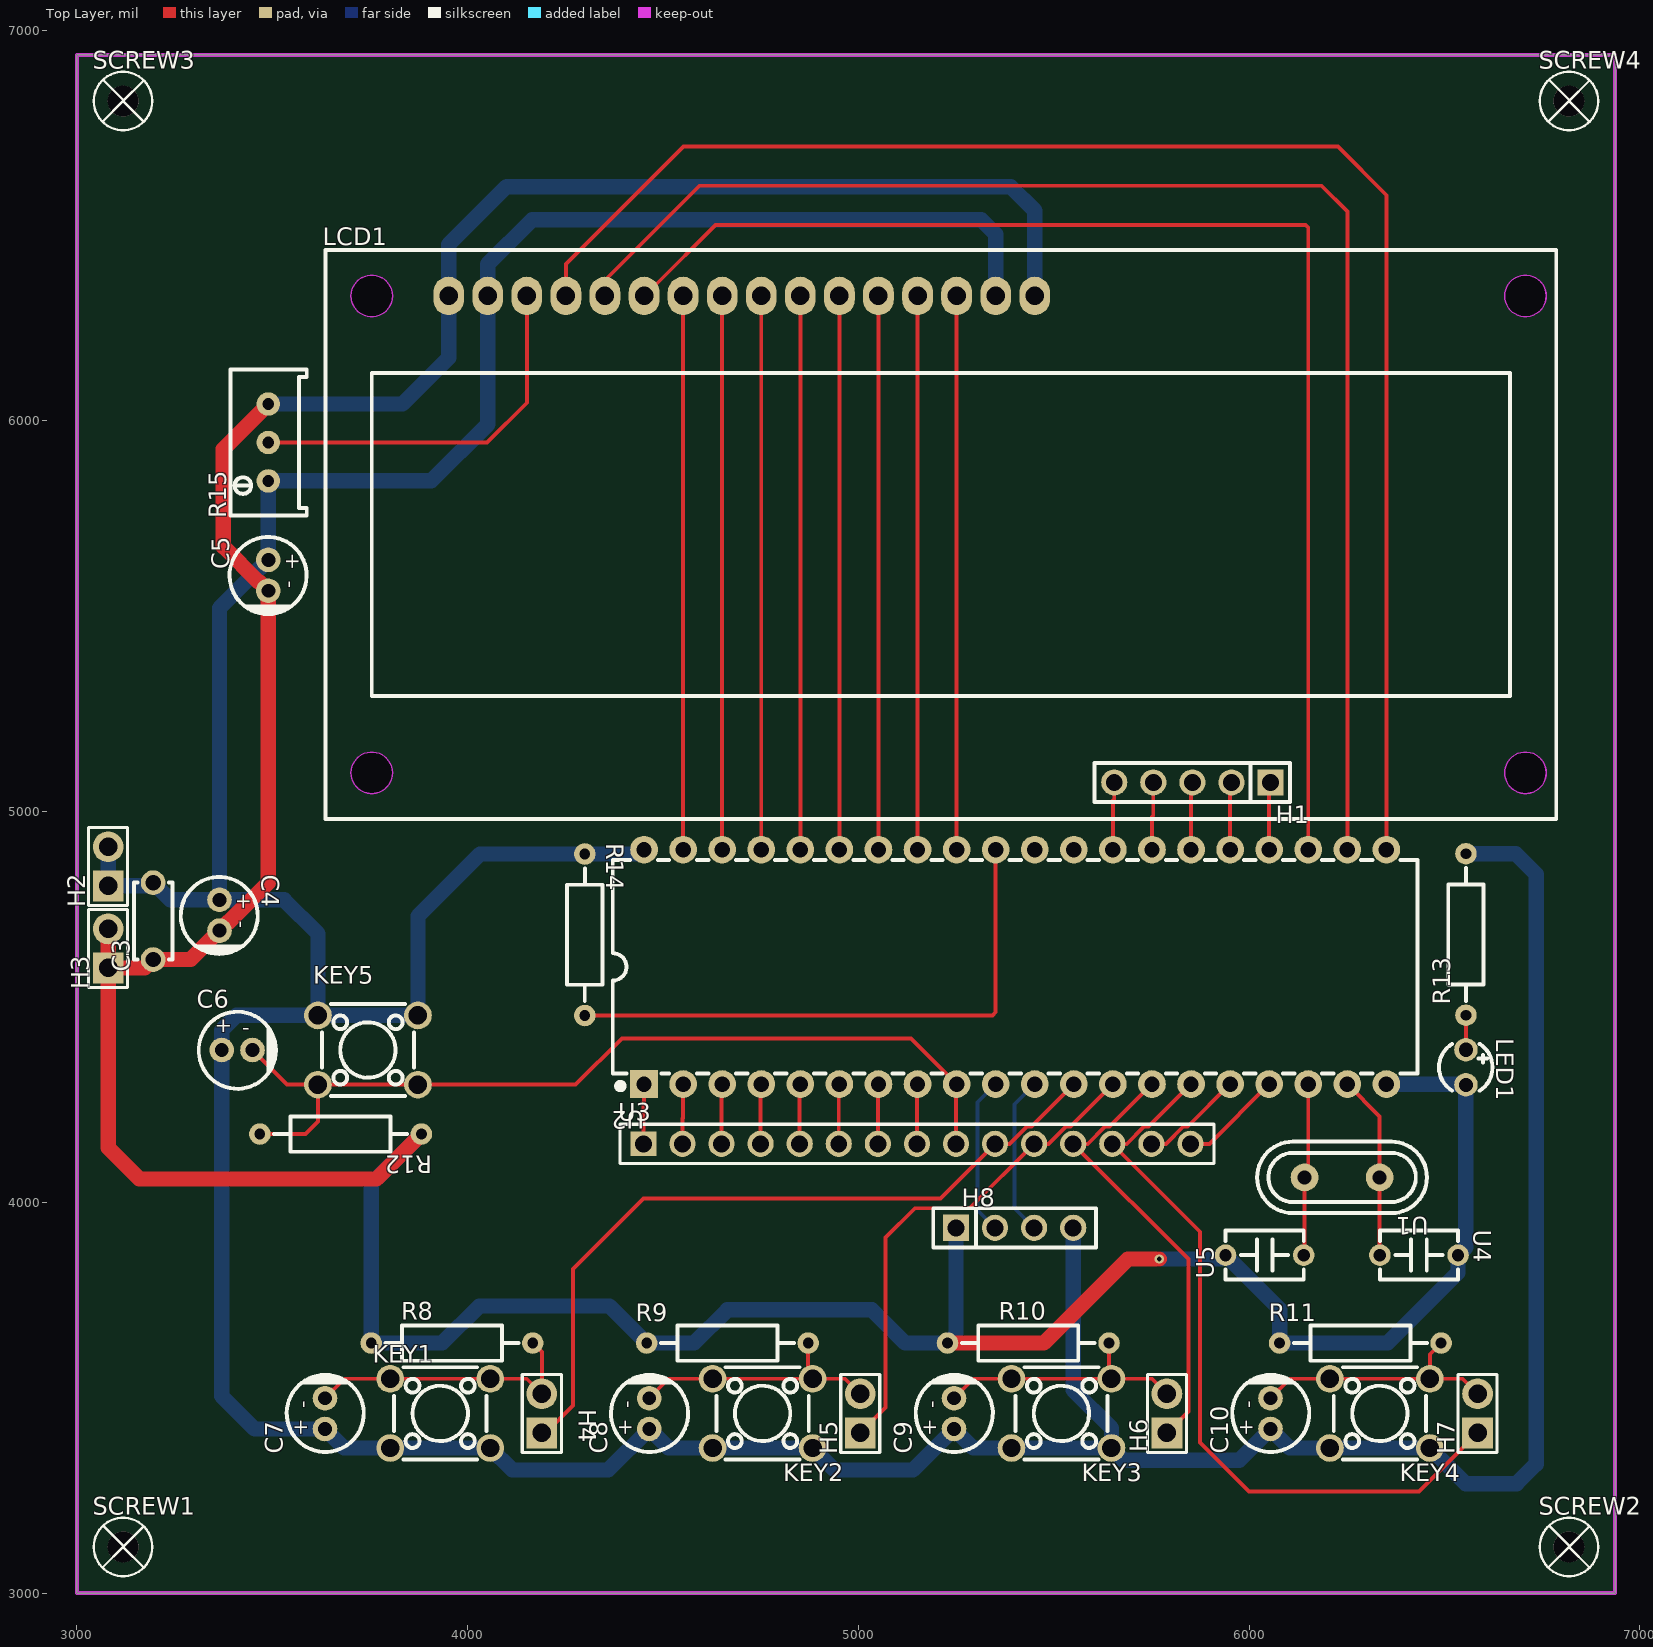
[diagram p0: Top Layer view]
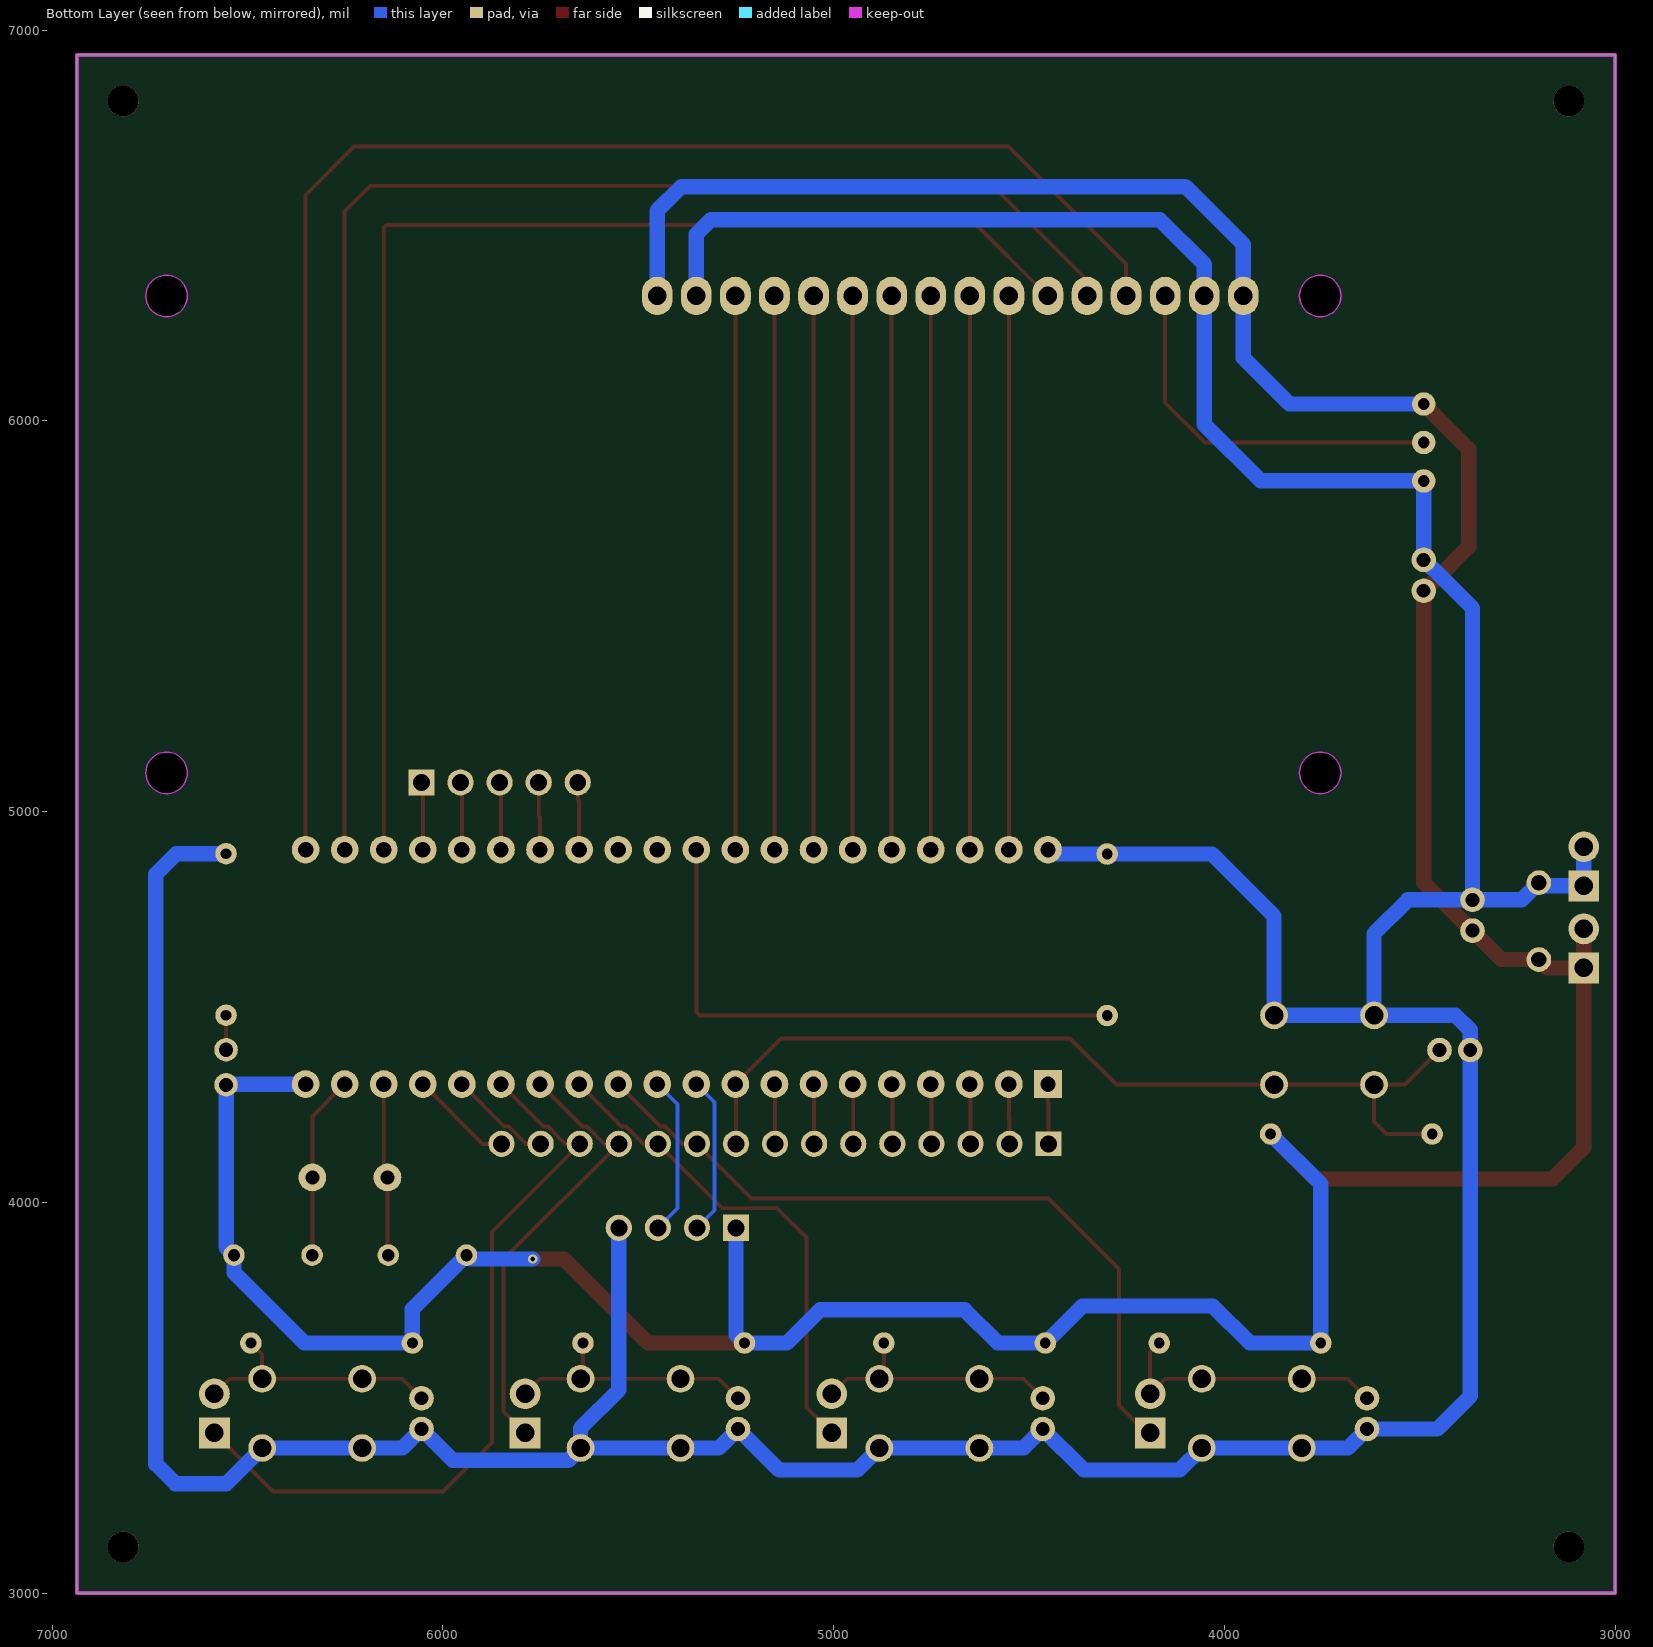
[diagram p1: Bottom Layer view, seen from below]
# Altium PCB MISC52019.pcbdoc
Units mil, origin at the board's own origin, x right, y up, seen from the top; angles counter-clockwise.
Board outline 3937.01 x 3937.01 mil, 2 copper layers (Top Layer, Bottom Layer), stack 62.206 mil thick; 40 components, 44 nets, 157 pads, 1 vias.

## Layer stack, top to bottom
Top Solder Mask Layer: solder mask 0.394, Dk 3.3
Top Layer: signal copper 1.379
Dielectric1: surface 59.449, FR4, Dk 4.5
Bottom Layer: signal copper 1.378
Bottom Solder Mask Layer: solder mask 0.394, Dk 3.3

## Board outline
3000,6937.01 3000,3000 6937.01,3000 6937.01,6937.01

## Design rules (kind name [scope] priority, off if disabled: settings)
BoardOutlineClearance copperThickness2oz_1 [All] p2 off: genericclearance=7.99 ignorepadtopadclearanceinfootprint=FALSE except(0: Arc-SplitContinuation Track-SplitContinuation SMDPad-SplitContinuation THPad-SplitContinuation Via-SplitContinuation Fill-SplitContinuation Region-SplitContinuation Poly-SplitContinuation Text-SplitContinuation Hole-SplitContinuation; 5.98: Arc-CutoutEdge Track-CutoutEdge SMDPad-CutoutEdge THPad-CutoutEdge Via-CutoutEdge Text-CutoutEdge; 6.9: Hole-OutlineEdge Hole-CutoutEdge; 10: Poly-OutlineEdge Poly-CutoutEdge; 11.81: Arc-OutlineEdge Track-OutlineEdge SMDPad-OutlineEdge THPad-OutlineEdge Via-OutlineEdge Fill-OutlineEdge Region-OutlineEdge Text-OutlineEdge Fill-CutoutEdge Region-CutoutEdge)
BoardOutlineClearance Plane_innerPlane_1 [All] p4 off: genericclearance=4.02 ignorepadtopadclearanceinfootprint=FALSE except(0: Arc-SplitContinuation Track-SplitContinuation SMDPad-SplitContinuation THPad-SplitContinuation Via-SplitContinuation Fill-SplitContinuation Region-SplitContinuation Poly-SplitContinuation Text-SplitContinuation Hole-SplitContinuation; 5.98: Arc-CutoutEdge Track-CutoutEdge SMDPad-CutoutEdge THPad-CutoutEdge Via-CutoutEdge Text-CutoutEdge; 6.9: Hole-OutlineEdge Hole-CutoutEdge; 10: Poly-OutlineEdge Poly-CutoutEdge; 11.81: Arc-OutlineEdge Track-OutlineEdge SMDPad-OutlineEdge THPad-OutlineEdge Via-OutlineEdge Fill-OutlineEdge Region-OutlineEdge Text-OutlineEdge Fill-CutoutEdge Region-CutoutEdge)
BoardOutlineClearance Copper_copperRegion_1 [All] p6 off: genericclearance=4.02 ignorepadtopadclearanceinfootprint=FALSE except(0: Arc-SplitContinuation Track-SplitContinuation SMDPad-SplitContinuation THPad-SplitContinuation Via-SplitContinuation Fill-SplitContinuation Region-SplitContinuation Poly-SplitContinuation Text-SplitContinuation Hole-SplitContinuation; 5.98: Arc-CutoutEdge Track-CutoutEdge SMDPad-CutoutEdge THPad-CutoutEdge Via-CutoutEdge Text-CutoutEdge; 6.9: Hole-OutlineEdge Hole-CutoutEdge; 10: Poly-OutlineEdge Poly-CutoutEdge; 11.81: Arc-OutlineEdge Track-OutlineEdge SMDPad-OutlineEdge THPad-OutlineEdge Via-OutlineEdge Fill-OutlineEdge Region-OutlineEdge Text-OutlineEdge Fill-CutoutEdge Region-CutoutEdge)
BoardOutlineClearance copperThickness1oz_1 [All] p8: genericclearance=4.02 ignorepadtopadclearanceinfootprint=FALSE except(0: Arc-SplitContinuation Track-SplitContinuation SMDPad-SplitContinuation THPad-SplitContinuation Via-SplitContinuation Fill-SplitContinuation Region-SplitContinuation Poly-SplitContinuation Text-SplitContinuation Hole-SplitContinuation; 5.98: Arc-CutoutEdge Track-CutoutEdge SMDPad-CutoutEdge THPad-CutoutEdge Via-CutoutEdge Text-CutoutEdge; 6.9: Hole-OutlineEdge Hole-CutoutEdge; 10: Poly-OutlineEdge Poly-CutoutEdge; 11.81: Arc-OutlineEdge Track-OutlineEdge SMDPad-OutlineEdge THPad-OutlineEdge Via-OutlineEdge Fill-OutlineEdge Region-OutlineEdge Text-OutlineEdge Fill-CutoutEdge Region-CutoutEdge)
Clearance copperThickness2oz [All] p1 off: gap=7.99 ignorepadtopadclearanceinfootprint=FALSE except(5.98: SMDPad-Track SMDPad-SMDPad THPad-Track SMDPad-THPad THPad-THPad Track-Via SMDPad-Via THPad-Via Via-Via Fill-SMDPad Region-SMDPad Fill-THPad Region-THPad Fill-Via Region-Via Fill-Fill Fill-Region Region-Region Arc-Track Arc-SMDPad Arc-THPad Arc-Via Fill-Arc Region-Arc Arc-Arc Text-Track SMDPad-Text Text-THPad Text-Via Fill-Text Region-Text Arc-Text Text-Text; 6.9: Hole-Track Hole-SMDPad Hole-THPad Hole-Via Fill-Hole Region-Hole Hole-Arc Hole-Text; 10: Poly-Track Poly-SMDPad Poly-THPad Poly-Via Poly-Fill Poly-Region Poly-Poly Poly-Arc Poly-Text Poly-Hole; 11.81: Fill-Track Region-Track)
Clearance Plane_innerPlane [All] p3 off: gap=4.02 ignorepadtopadclearanceinfootprint=FALSE except(5.98: SMDPad-Track SMDPad-SMDPad THPad-Track SMDPad-THPad THPad-THPad Track-Via SMDPad-Via THPad-Via Via-Via Fill-SMDPad Region-SMDPad Fill-THPad Region-THPad Fill-Via Region-Via Fill-Fill Fill-Region Region-Region Arc-Track Arc-SMDPad Arc-THPad Arc-Via Fill-Arc Region-Arc Arc-Arc Text-Track SMDPad-Text Text-THPad Text-Via Fill-Text Region-Text Arc-Text Text-Text; 6.9: Hole-Track Hole-SMDPad Hole-THPad Hole-Via Fill-Hole Region-Hole Hole-Arc Hole-Text; 10: Poly-Track Poly-SMDPad Poly-THPad Poly-Via Poly-Fill Poly-Region Poly-Poly Poly-Arc Poly-Text Poly-Hole; 11.81: Fill-Track Region-Track)
Clearance Copper_copperRegion [All] p5 off: gap=4.02 ignorepadtopadclearanceinfootprint=FALSE except(5.98: SMDPad-Track SMDPad-SMDPad THPad-Track SMDPad-THPad THPad-THPad Track-Via SMDPad-Via THPad-Via Via-Via Fill-SMDPad Region-SMDPad Fill-THPad Region-THPad Fill-Via Region-Via Fill-Fill Fill-Region Region-Region Arc-Track Arc-SMDPad Arc-THPad Arc-Via Fill-Arc Region-Arc Arc-Arc Text-Track SMDPad-Text Text-THPad Text-Via Fill-Text Region-Text Arc-Text Text-Text; 6.9: Hole-Track Hole-SMDPad Hole-THPad Hole-Via Fill-Hole Region-Hole Hole-Arc Hole-Text; 10: Poly-Track Poly-SMDPad Poly-THPad Poly-Via Poly-Fill Poly-Region Poly-Poly Poly-Arc Poly-Text Poly-Hole; 11.81: Fill-Track Region-Track)
Clearance copperThickness1oz [All] p7: gap=4.02 ignorepadtopadclearanceinfootprint=FALSE except(5.98: SMDPad-Track SMDPad-SMDPad THPad-Track SMDPad-THPad THPad-THPad Track-Via SMDPad-Via THPad-Via Via-Via Fill-SMDPad Region-SMDPad Fill-THPad Region-THPad Fill-Via Region-Via Fill-Fill Fill-Region Region-Region Arc-Track Arc-SMDPad Arc-THPad Arc-Via Fill-Arc Region-Arc Arc-Arc Text-Track SMDPad-Text Text-THPad Text-Via Fill-Text Region-Text Arc-Text Text-Text; 6.9: Hole-Track Hole-SMDPad Hole-THPad Hole-Via Fill-Hole Region-Hole Hole-Arc Hole-Text; 10: Poly-Track Poly-SMDPad Poly-THPad Poly-Via Poly-Fill Poly-Region Poly-Poly Poly-Arc Poly-Text Poly-Hole; 11.81: Fill-Track Region-Track)
DiffPairsRouting differentialPair [All] p1: maxlimit=6 minlimit=6 mostfreqgap=6 toplayer_minwidth=5 toplayer_prefwidth=10 toplayer_maxwidth=100 toplayer_mingap=6 toplayer_prefgap=6 toplayer_maxgap=6 bottomlayer_minwidth=5 bottomlayer_prefwidth=10 bottomlayer_maxwidth=100 bottomlayer_mingap=6 bottomlayer_prefgap=6 bottomlayer_maxgap=6 maxuncoupledlength=10
HoleToHoleClearance otherClearance [All] p1: gap=11.81 allowstackedmicrovias=TRUE
Length netLength [All] p1: minlimit=0 maxlimit=0
PasteMaskExpansion pasteMaskExpansion [All] p1: expansion=0
PlaneConnect innerPlane [All] p1: planeconnectstyle=Relief reliefexpansion=20 reliefentries=4 reliefconductorwidth=10 reliefairgap=10
PolygonConnect copperRegion [All] p1: connectstyle=Relief reliefconductorwidth=10 reliefentries=4 polygonreliefangle="90 Angle" airgapwidth=10 via.connectstyle=Relief via.reliefconductorwidth=10 via.reliefentries=4 via.polygonreliefangle="90 Angle" via.airgapwidth=10
RoutingVias viaSize [All] p1: holewidth=12.01 width=24.02 viastyle="Through Hole" minholewidth=11.81 minwidth=19.68 maxholewidth=248.03 maxwidth=393.7
SolderMaskExpansion solderMaskExpansion [IsVia] p1: expansion=-1000 istentingtop=TRUE
SolderMaskExpansion solderMaskExpansion [All] p2: expansion=2 istentingtop=FALSE
Width copperThickness2oz_2 [All] p1 off: maxlimit=100 minlimit=8 preferedwidth=10
Width copperThickness1oz_2 [All] p2: maxlimit=100 minlimit=5 preferedwidth=10

## Components (designator, comment, footprint, x,y, rotation, side; value= is the part's Value field where it differs from the comment)
C3 "100nF" CAP-TH_L5.0-W2.5-P5.00-D1.0 3195,4720 r90 top
C4 "10uF" CAP-TH_BD5.0-P2.00-D0.5-FD-A 3365,4735 r270 top
C5 "10uF" CAP-TH_BD5.0-P2.00-D0.5-FD-A 3490,5605 r270 top
C6 "10uF" CAP-TH_BD5.0-P2.00-D0.5-FD-A 3410,4390 r0 top
C7 "10uF" CAP-TH_BD5.0-P2.00-D0.5-FD-A 3635,3459.5 r90 top
C8 "10uF" CAP-TH_BD5.0-P2.00-D0.5-FD-A 4465,3459.5 r90 top
C9 "10uF" CAP-TH_BD5.0-P2.00-D0.5-FD-A 5245,3459.5 r90 top
C10 "10uF" CAP-TH_BD5.0-P2.00-D0.5-FD-A 6055,3459.5 r90 top
H1 "PZ254V-11-05P" HDR-TH_5P-P2.54-V-M 5855,5075 r180 top
H2 "PZ254V-11-02P" HDR-TH_2P-P2.54-V-M 3080,4860 r90 top
H3 "PZ254V-11-02P" HDR-TH_2P-P2.54-V-M 3080,4650 r90 top
H4 "PZ254V-11-02P" HDR-TH_2P-P2.54-V-M 4190,3460 r90 top
H5 "PZ254V-11-02P" HDR-TH_2P-P2.54-V-M 5005,3460 r90 top
H6 "PZ254V-11-02P" HDR-TH_2P-P2.54-V-M 5790,3460 r90 top
H7 "PZ254V-11-02P" HDR-TH_2P-P2.54-V-M 6585,3460 r90 top
H8 "" HDR-TH_4P-P2.54-V-F 5400,3935 r0 top
KEY1 "" SW-TH_4P-L6.0-W6.0-P4.50-LS6.5 3930,3460 r180 top
KEY2 "" SW-TH_4P-L6.0-W6.0-P4.50-LS6.5 4755,3460 r180 top
KEY3 "" SW-TH_4P-L6.0-W6.0-P4.50-LS6.5 5520,3460 r180 top
KEY4 "" SW-TH_4P-L6.0-W6.0-P4.50-LS6.5 6335,3460 r180 top
KEY5 "" SW-TH_4P-L6.0-W6.0-P4.50-LS6.5 3745,4390 r180 top
LCD1 "LCM1602K-NSW-BBW" MODULE-TH_LCM1602K 4701.61,6320 r0 top
LED1 "3A2RUD" LED-TH_BD3.5-P2.28_3A2RUC 6555.18,4345.82 r270 top
R8 "10kΩ" RES-TH_BD2.3-L6.5-P10.50-D0.5 3960,3640 r0 top
R9 "10kΩ" RES-TH_BD2.3-L6.5-P10.50-D0.5 4665,3640 r0 top
R10 "10kΩ" RES-TH_BD2.3-L6.5-P10.50-D0.5 5435,3640 r0 top
R11 "10kΩ" RES-TH_BD2.3-L6.5-P10.50-D0.5 6285,3640 r0 top
R12 "10kΩ" RES-TH_BD2.3-L6.5-P10.50-D0.5 3675,4175 r180 top
R13 "10kΩ" RES-TH_BD2.3-L6.5-P10.50-D0.5 6555.18,4685.82 r90 top
R14 "10kΩ" RES-TH_BD2.3-L6.5-P10.50-D0.5 4300,4685 r270 top
R15 "10kΩ" RES-ADJ-TH_3P-L10.0-W10.0-P2.50-L 3490,5945 r90 top
SCREW1 "" M2螺丝 3118.11,3118.11 r0 top
SCREW2 "" M2螺丝 6818.9,3118.11 r0 top
SCREW3 "" M2螺丝 3118.11,6818.9 r0 top
SCREW4 "" M2螺丝 6818.9,6818.9 r0 top
U1 "12MHz" HC-49S_L11.0-W4.7-P4.88 6238.18,4063.91 r180 top
U2 "STC89C516RD+40I-PDIP40" DIP-40_L52.3-W13.9-P2.54-LS15.2-BL 5401.61,4602.88 r0 top
U3 "ZX-PM2.54-1-15PY" HDR-TH_15P-P2.54-V-F 5150,4150 r0 top
U4 "33pF" CAP-TH_L5.0-W2.5-P5.08-D0.7 6435,3865 r180 top
U5 "33pF" CAP-TH_L5.0-W2.5-P5.08-D0.7 6040,3865 r0 top

## Footprints (in the part's own frame and the unit in brackets; to place one, negate y for a bottom-side part, rotate by r counter-clockwise, add the part's x,y. Pads: shape width x height; smd on the part's side, far side on the other; paste and mask are expansions set on the pad)
CAP-TH_BD5.0-P2.00-D0.5-FD-A [mm]
  round 1.6 hole 0.9 paste+0 mask+0.05: 1(-1,0) 2(1,0)
  silkscreen extent -2.49,-2.52 2.6,2.49
CAP-TH_L5.0-W2.5-P5.00-D1.0 [mm]
  round 1.6 hole 1: 1(-2.5,0) 2(2.5,0)
  silkscreen extent -2.5,-1.27 2.5,1.25
CAP-TH_L5.0-W2.5-P5.08-D0.7 [mm]
  round 1.4 hole 0.8: 1(-2.54,0) 2(2.54,0)
  silkscreen extent -2.54,-1.59 2.54,1.59
DIP-40_L52.3-W13.9-P2.54-LS15.2-BL [mm]
  rect 1.8x1.8 hole 1: 1(-24.13,-7.62)
  round 1.8 hole 1: 2(-21.59,-7.62) 3(-19.05,-7.62) 4(-16.51,-7.62) 5(-13.97,-7.62) 6(-11.43,-7.62) 7(-8.89,-7.62) 8(-6.35,-7.62) 9(-3.81,-7.62) 10(-1.27,-7.62) 11(1.27,-7.62) 12(3.81,-7.62) 13(6.35,-7.62) 14(8.89,-7.62) 15(11.43,-7.62) 16(13.97,-7.62) 17(16.51,-7.62) 18(19.05,-7.62) 19(21.59,-7.62) 20(24.13,-7.62) 21(24.13,7.62) 22(21.59,7.62) 23(19.05,7.62) 24(16.51,7.62) 25(13.97,7.62) 26(11.43,7.62) 27(8.89,7.62) 28(6.35,7.62) 29(3.81,7.62) 30(1.27,7.62) 31(-1.27,7.62) 32(-3.81,7.62) 33(-6.35,7.62) 34(-8.89,7.62) 35(-11.43,7.62) 36(-13.97,7.62) 37(-16.51,7.62) 38(-19.05,7.62) 39(-21.59,7.62) 40(-24.13,7.62)
  silkscreen extent -26.16,-7.95 26.16,6.93
HC-49S_L11.0-W4.7-P4.88 [mm]
  round 1.8 hole 0.9: 1(-2.44,0) 2(2.44,0)
  silkscreen extent -5.52,-2.32 5.52,2.33
HDR-TH_2P-P2.54-V-M [mm]
  rect 2x2 hole 1.2: 1(-1.27,0)
  round 2 hole 1.2: 2(1.27,0)
  silkscreen extent -2.54,-1.27 2.54,1.27
HDR-TH_4P-P2.54-V-F [mm]
  rect 1.7x1.7 hole 1.1: 1(-3.81,0)
  round 1.7 hole 1.1: 2(-1.27,0) 3(1.27,0) 4(3.81,0)
  silkscreen extent -5.29,-1.27 5.29,1.27
HDR-TH_5P-P2.54-V-M [mm]
  rect 1.7x1.7 hole 1.1: 1(-5.08,0)
  round 1.7 hole 1.1: 2(-2.54,0) 3(0,0) 4(2.54,0) 5(5.08,0)
  silkscreen extent -6.35,-1.27 6.35,1.27
HDR-TH_15P-P2.54-V-F [mm]
  rect 1.7x1.575 hole 1.1: 1(-17.78,0)
  round 1.7 hole 1.1: 2(-15.24,0) 3(-12.7,0) 4(-10.16,0) 5(-7.62,0) 6(-5.08,0) 7(-2.54,0) 8(0,0) 9(2.54,0) 10(5.08,0) 11(7.62,0) 12(10.16,0) 13(12.7,0) 14(15.24,0) 15(17.78,0)
  silkscreen extent -19.3,-1.27 19.3,1.27
LED-TH_BD3.5-P2.28_3A2RUC [mil]
  round 60 hole 36: 1(44.88,0) 2(-44.88,0)
  silkscreen extent -60,-69 60,68
M2螺丝 [mm]
  round 2 hole 2: 1(0,0)
  silkscreen extent -1.9,-1.9 1.9,1.9
MODULE-TH_LCM1602K [mm]
  oval 2x2.5 hole 1.2: 1(-19.05,0) 2(-16.51,0) 3(-13.97,0) 4(-11.43,0) 5(-8.89,0) 6(-6.35,0) 7(-3.81,0) 8(-1.27,0) 9(1.27,0) 10(3.81,0) 11(6.35,0) 12(8.89,0) 13(11.43,0) 14(13.97,0) 15(16.51,0) 16(19.05,0)
  Board Outline Layer circle w0.003: c-24.051,0 r1.35
  Board Outline Layer circle w0.003: c50.95,0 r1.35
  Board Outline Layer circle w0.003: c50.95,-31.001 r1.35
  Board Outline Layer circle w0.003: c-24.051,-31.001 r1.35
  Board Outline Layer region: -22.701,0 -22.835,-0.586 -23.21,-1.055 -23.751,-1.316 -24.352,-1.316 -24.893,-1.055 -25.268,-0.586 -25.401,0 -25.401,0 -25.268,0.586 -24.893,1.055 -24.352,1.316 -23.751,1.316 -23.21,1.055 -22.835,0.586 -22.701,0
  Board Outline Layer region: -22.701,0 -22.711,-0.163 -22.74,-0.323 -22.789,-0.479 -22.856,-0.627 -22.94,-0.767 -23.041,-0.895 -23.156,-1.01 -23.284,-1.111 -23.424,-1.195 -23.573,-1.262 -23.728,-1.311 -23.889,-1.34 -24.051,-1.35 -24.214,-1.34 -24.374,-1.311 -24.53,-1.262 -24.679,-1.195 -24.818,-1.111 -24.946,-1.01 -25.062,-0.895 -25.162,-0.767 -25.247,-0.627 -25.314,-0.479 -25.362,-0.323 -25.391,-0.163 -25.401,0 -25.391,0.163 -25.362,0.323 -25.314,0.479 -25.247,0.627 -25.162,0.767 -25.062,0.895 -24.946,1.01 -24.818,1.111 -24.679,1.195 -24.53,1.262 -24.374,1.311 -24.214,1.34 -24.051,1.35 -23.889,1.34 -23.728,1.311 -23.573,1.262 -23.424,1.195 -23.284,1.111 -23.156,1.01 -23.041,0.895 -22.94,0.767 -22.856,0.627 -22.789,0.479 -22.74,0.323 -22.711,0.163
  Board Outline Layer region: 52.3,0 52.166,-0.586 51.792,-1.055 51.25,-1.316 50.649,-1.316 50.108,-1.055 49.734,-0.586 49.6,0 49.6,0 49.734,0.586 50.108,1.055 50.649,1.316 51.25,1.316 51.792,1.055 52.166,0.586 52.3,0
  Board Outline Layer region: 52.3,0 52.29,-0.163 52.261,-0.323 52.212,-0.479 52.145,-0.627 52.061,-0.767 51.96,-0.895 51.845,-1.01 51.717,-1.111 51.577,-1.195 51.429,-1.262 51.273,-1.311 51.113,-1.34 50.95,-1.35 50.787,-1.34 50.627,-1.311 50.471,-1.262 50.322,-1.195 50.183,-1.111 50.055,-1.01 49.939,-0.895 49.839,-0.767 49.754,-0.627 49.688,-0.479 49.639,-0.323 49.61,-0.163 49.6,0 49.61,0.163 49.639,0.323 49.688,0.479 49.754,0.627 49.839,0.767 49.939,0.895 50.055,1.01 50.183,1.111 50.322,1.195 50.471,1.262 50.627,1.311 50.787,1.34 50.95,1.35 51.113,1.34 51.273,1.311 51.429,1.262 51.577,1.195 51.717,1.111 51.845,1.01 51.96,0.895 52.061,0.767 52.145,0.627 52.212,0.479 52.261,0.323 52.29,0.163
  Board Outline Layer region: 52.3,-31.001 52.166,-31.586 51.792,-32.056 51.25,-32.317 50.649,-32.317 50.108,-32.056 49.734,-31.586 49.6,-31.001 49.6,-31.001 49.734,-30.415 50.108,-29.945 50.649,-29.685 51.25,-29.685 51.792,-29.945 52.166,-30.415 52.3,-31.001
  Board Outline Layer region: 52.3,-31.001 52.29,-31.163 52.261,-31.324 52.212,-31.479 52.145,-31.628 52.061,-31.768 51.96,-31.896 51.845,-32.011 51.717,-32.112 51.577,-32.196 51.429,-32.263 51.273,-32.311 51.113,-32.341 50.95,-32.351 50.787,-32.341 50.627,-32.311 50.471,-32.263 50.322,-32.196 50.183,-32.112 50.055,-32.011 49.939,-31.896 49.839,-31.768 49.754,-31.628 49.688,-31.479 49.639,-31.324 49.61,-31.163 49.6,-31.001 49.61,-30.838 49.639,-30.678 49.688,-30.522 49.754,-30.373 49.839,-30.234 49.939,-30.105 50.055,-29.99 50.183,-29.89 50.322,-29.805 50.471,-29.738 50.627,-29.69 50.787,-29.661 50.95,-29.651 51.113,-29.661 51.273,-29.69 51.429,-29.738 51.577,-29.805 51.717,-29.89 51.845,-29.99 51.96,-30.105 52.061,-30.234 52.145,-30.373 52.212,-30.522 52.261,-30.678 52.29,-30.838
  Board Outline Layer region: -22.701,-31.001 -22.835,-31.586 -23.21,-32.056 -23.751,-32.317 -24.352,-32.317 -24.893,-32.056 -25.268,-31.586 -25.401,-31.001 -25.401,-31.001 -25.268,-30.415 -24.893,-29.945 -24.352,-29.685 -23.751,-29.685 -23.21,-29.945 -22.835,-30.415 -22.701,-31.001
  Board Outline Layer region: -22.701,-31.001 -22.711,-31.163 -22.74,-31.324 -22.789,-31.479 -22.856,-31.628 -22.94,-31.768 -23.041,-31.896 -23.156,-32.011 -23.284,-32.112 -23.424,-32.196 -23.573,-32.263 -23.728,-32.311 -23.889,-32.341 -24.051,-32.351 -24.214,-32.341 -24.374,-32.311 -24.53,-32.263 -24.679,-32.196 -24.818,-32.112 -24.946,-32.011 -25.062,-31.896 -25.162,-31.768 -25.247,-31.628 -25.314,-31.479 -25.362,-31.324 -25.391,-31.163 -25.401,-31.001 -25.391,-30.838 -25.362,-30.678 -25.314,-30.522 -25.247,-30.373 -25.162,-30.234 -25.062,-30.105 -24.946,-29.99 -24.818,-29.89 -24.679,-29.805 -24.53,-29.738 -24.374,-29.69 -24.214,-29.661 -24.051,-29.651 -23.889,-29.661 -23.728,-29.69 -23.573,-29.738 -23.424,-29.805 -23.284,-29.89 -23.156,-29.99 -23.041,-30.105 -22.94,-30.234 -22.856,-30.373 -22.789,-30.522 -22.74,-30.678 -22.711,-30.838
  Multi-Layer board cut-out: -22.701,0 -22.835,-0.586 -23.21,-1.055 -23.751,-1.316 -24.352,-1.316 -24.893,-1.055 -25.268,-0.586 -25.401,0 -25.401,0 -25.268,0.586 -24.893,1.055 -24.352,1.316 -23.751,1.316 -23.21,1.055 -22.835,0.586 -22.701,0
  Multi-Layer board cut-out: 52.3,0 52.166,-0.586 51.792,-1.055 51.25,-1.316 50.649,-1.316 50.108,-1.055 49.734,-0.586 49.6,0 49.6,0 49.734,0.586 50.108,1.055 50.649,1.316 51.25,1.316 51.792,1.055 52.166,0.586 52.3,0
  Multi-Layer board cut-out: 52.3,-31.001 52.166,-31.586 51.792,-32.056 51.25,-32.317 50.649,-32.317 50.108,-32.056 49.734,-31.586 49.6,-31.001 49.6,-31.001 49.734,-30.415 50.108,-29.945 50.649,-29.685 51.25,-29.685 51.792,-29.945 52.166,-30.415 52.3,-31.001
  Multi-Layer board cut-out: -22.701,-31.001 -22.835,-31.586 -23.21,-32.056 -23.751,-32.317 -24.352,-32.317 -24.893,-32.056 -25.268,-31.586 -25.401,-31.001 -25.401,-31.001 -25.268,-30.415 -24.893,-29.945 -24.352,-29.685 -23.751,-29.685 -23.21,-29.945 -22.835,-30.415 -22.701,-31.001
  silkscreen extent -27.05,-34 52.95,3
RES-ADJ-TH_3P-L10.0-W10.0-P2.50-L [mil]
  round 60 hole 30: 1(-98.43,0) 2(0,0) 3(98.43,0)
  silkscreen extent -187,-98 187,96
RES-TH_BD2.3-L6.5-P10.50-D0.5 [mm]
  round 1.4 hole 0.7: 1(-5.25,0) 2(5.25,0)
  silkscreen extent -4.32,-1.15 4.32,1.15
SW-TH_4P-L6.0-W6.0-P4.50-LS6.5 [mm]
  round 1.8 hole 1.2: 1(-3.25,2.25) 2(3.25,2.25) 3(-3.25,-2.25) 4(3.25,-2.25)
  silkscreen extent -3,-3 3,3

## Via types
v1: diameter 24.02, hole 12, Top Layer to Bottom Layer, 1 vias

## Nets (pads, with @x,y where several pads share a name; then routed paths per layer and width w, separated by ;. In a path a pad name is that pad's centre, name@x,y a point inside that pad or via, vN(x,y) a via of type N, cw(c..) or ccw(c..) an arc to the next point about the centre after c; other vN are vias at no path point)
$1N854: LED1.2 R13.1 | length 88.4
  Top Layer w10: LED1.2 R13.1
$1N1184: R14.2 U2.31 | length 1471.3
  Top Layer w10: R14.2 5343.31,4478.31 5351.61,4486.61 U2.31
$1N2217: LCD1.3 R15.2 | length 977.1
  Top Layer w10: R15.2 4050.01,5945.01 4151.61,6046.61 LCD1.3
$1N3173: C7.2 H4.2 KEY1.3 KEY1.4 R8.2 | length 731.2
  Top Layer w10: C7.2 3684.71,3548.58 KEY1.4 KEY1.3 4151.42,3548.58 H4.2 4190,3616.69 R8.2
$1N3440: C8.2 H5.2 KEY2.3 KEY2.4 R9.2 | length 672.7
  Top Layer w10: C8.2 4514.71,3548.58 KEY2.4 KEY2.3 ; R9.2 4871.69,3559.84 KEY2.3 ; H5.2 4966.42,3548.58 KEY2.3
$1N3634: C9.2 H6.2 KEY3.3 KEY3.4 R10.2 | length 675.6
  Top Layer w10: C9.2 5294.71,3548.58 KEY3.4 KEY3.3 ; R10.2 5641.69,3554.84 KEY3.3 ; H6.2 5751.42,3548.58 KEY3.3
$1N3828: C10.2 H7.2 KEY4.3 KEY4.4 R11.2 | length 669.9
  Top Layer w10: C10.2 6104.71,3548.58 KEY4.4 KEY4.3 ; R11.2 6462.95,3611.26 KEY4.3 ; H7.2 6546.42,3548.58 KEY4.3
+5V: C3.2 C4.1 C5.1 C6.1 C7.1 C8.1 C9.1 C10.1 H2.1 H2.2 H8.4 KEY1.1 KEY1.2 KEY2.1 KEY2.2 KEY3.1 KEY3.2 KEY4.1 KEY4.2 KEY5.3 KEY5.4 LCD1.2 LCD1.15 R13.2 R14.1 R15.1 U2.40 | length 12973.4
  Bottom Layer w39.37: H2.2 H2.1 3186.57,4810 C3.2 3239.05,4774.37 C4.1 ; U2.40 4440.42,4891.69 R14.1 4031.69,4891.69 3872.95,4732.95 KEY5.3 KEY5.4 ; LCD1.15 5351.61,6478.39 5315,6515 4165,6515 4051.61,6401.61 LCD1.2 4051.61,5991.61 3906.57,5846.57 R15.1 C5.1 3468.42,5622.8 3466.32,5622.8 3365,5521.47 C4.1 ; H8.4 5550,3520 5647.95,3422.05 KEY3.1 ; R13.2 6682.49,4892.51 6735,4840 6735,3330 6685,3280 6554.37,3280 KEY4.1 KEY4.2 6103.71,3371.42 C10.1 5974.87,3340 5679.37,3340 KEY3.1 ; C4.1 3530.63,4774.37 3617.05,4687.95 KEY5.4 ; KEY5.4 3408.58,4478.58 3370.63,4440.63 C6.1 3370.63,3504.37 3454.87,3420.13 C7.1 3683.71,3371.42 KEY1.2 KEY1.1 4114.37,3315 4359.87,3315 C8.1 4513.71,3371.42 KEY2.2 KEY2.1 4939.37,3315 5139.87,3315 C9.1 5293.71,3371.42 KEY3.2 KEY3.1
GND: C3.1 C4.2 C5.2 H3.1 H3.2 H8.1 LCD1.1 LCD1.16 LED1.1 R8.1 R9.1 R10.1 R11.1 R12.1 R15.3 U2.20 U4.1 U5.1 | length 10698.7
  Top Layer w39.37: H3.2 H3.1 ; R15.3 3375,5928.43 3375,5678.52 3466.32,5587.2 3468.42,5587.2 C5.2 3490,4818.53 3388.67,4717.2 3386.57,4717.2 C4.2 3290.94,4621.57 C3.1 3173.43,4600 H3.1 ; R12.1 3766.69,4060 3160,4060 3080,4140 H3.1 ; R10.1 5475,3640 5690,3855 v1(5770,3855)
  Bottom Layer w39.37: R15.3 3833.43,6043.43 3951.61,6161.61 LCD1.1 3951.61,6451.61 4100,6600 5390,6600 5451.61,6538.39 LCD1.16 ; R12.1 3753.31,4046.62 R8.1 3935,3640 4030,3735 4363.31,3735 R9.1 4580,3640 4665,3725 5035,3725 5120,3640 R10.1 5250,3661.69 H8.1 ; v1(5770,3855) 5930,3855 U5.1 6078.31,3726.69 R11.1 6355,3640 6535,3820 U4.1 6555.18,3885.18 LED1.1 6553.24,4302.88 U2.20
P00: LCD1.7 U2.39 | length 1417.1
  Top Layer w10: U2.39 LCD1.7
P01: LCD1.8 U2.38 | length 1417.1
  Top Layer w10: U2.38 LCD1.8
P02: LCD1.9 U2.37 | length 1417.1
  Top Layer w10: U2.37 LCD1.9
P03: LCD1.10 U2.36 | length 1417.1
  Top Layer w10: U2.36 LCD1.10
P04: LCD1.11 U2.35 | length 1417.1
  Top Layer w10: U2.35 LCD1.11
P05: LCD1.12 U2.34 | length 1417.1
  Top Layer w10: U2.34 LCD1.12
P06: LCD1.13 U2.33 | length 1417.1
  Top Layer w10: U2.33 LCD1.13
P07: LCD1.14 U2.32 | length 1417.1
  Top Layer w10: U2.32 LCD1.14
P10: U2.1 U3.1 | length 153.5
  Top Layer w10: U3.1 4450,4255.83 4451.61,4257.44 U2.1
P11: U2.2 U3.2 | length 153.5
  Top Layer w10: U3.2 4550,4214.41 4551.61,4216.02 U2.2
P12: U2.3 U3.3 | length 153.5
  Top Layer w10: U3.3 4650,4301.27 U2.3
P13: U2.4 U3.4 | length 153.5
  Top Layer w10: U3.4 4750,4301.27 U2.4
P14: U2.5 U3.5 | length 153.5
  Top Layer w10: U3.5 4850,4301.27 U2.5
P15: U2.6 U3.6 | length 153.5
  Top Layer w10: U3.6 4950,4301.27 U2.6
P16: U2.7 U3.7 | length 153.5
  Top Layer w10: U3.7 5050,4301.27 U2.7
P17: U2.8 U3.8 | length 153.5
  Top Layer w10: U3.8 5150,4301.27 U2.8
P20: LCD1.4 U2.21 | length 4032.5
  Top Layer w10: LCD1.4 4251.61,6401.61 4552.07,6702.07 6227.38,6702.07 6351.61,6577.84 U2.21
P21: LCD1.5 U2.22 | length 3701.1
  Top Layer w10: LCD1.5 4351.61,6360.19 4593.49,6602.07 6185.96,6602.07 6251.61,6536.42 U2.22
P22: LCD1.6 U2.23 | length 3335.9
  Top Layer w10: LCD1.6@4476.42,6343.58 4634.91,6502.07 6144.54,6502.07 6151.61,6495 U2.23
P23: H1.1 U2.24 | length 173.5
  Top Layer w10: U2.24 6051.61,5071.61 H1.1
P24: H1.2 U2.25 | length 173.5
  Top Layer w10: U2.25 5951.61,5071.61 H1.2
P25: H1.3 U2.26 | length 173.5
  Top Layer w10: U2.26 5851.61,5071.61 H1.3
P26: H1.4 U2.27 | length 173.5
  Top Layer w10: U2.27 5751.61,4986.72 5755,4990.11 H1.4
P27: H1.5 U2.28 | length 173.5
  Top Layer w10: U2.28 5651.61,5028.14 5655,5031.54 H1.5
P30: H8.2 U2.10 | length 405.8
  Bottom Layer w10: H8.2 5305,3980 5305,4256.27 U2.10
P31: H8.3 U2.11 | length 410
  Bottom Layer w10: H8.3 5400,3985 5400,4251.27 U2.11
P32: H4.1 U2.12 U3.10 | length 1936.5
  Top Layer w10: H4.1 4200,3410 4270,3480 4270,3830 4450,4010 5210,4010 U3.10 5387.14,4150 5431.59,4194.45 5443.18,4194.45 U2.12
P33: H5.1 U2.13 U3.11 | length 1271.3
  Top Layer w10: H5.1 5070,3475 5070,3910 5145,3985 5285,3985 U3.11 5487.14,4150 5531.59,4194.45 5543.18,4194.45 U2.13
P34: H6.1 U2.14 U3.12 | length 1149.9
  Top Layer w10: U2.14 5643.18,4194.45 5631.59,4194.45 5587.14,4150 U3.12 5845,3855 5845,3465 H6.1
P35: H7.1 U2.15 U3.13 | length 1947
  Top Layer w10: U2.15 5743.18,4194.45 5731.59,4194.45 5687.14,4150 U3.13 5875,3925 5875,3385 6000,3260 6435,3260 H7.1
P36: U2.16 U3.14 | length 264.9
  Top Layer w10: U3.14 5787.14,4150 5831.59,4194.45 5843.18,4194.45 U2.16
P37: U2.17 U3.15 | length 264.9
  Top Layer w10: U3.15 5898.73,4150 U2.17
RST: C6.2 KEY5.1 KEY5.2 R12.2 U2.9 U3.9 | length 2346.5
  Top Layer w10: C6.2 3537.95,4301.42 KEY5.2 ; R12.2 3585,4175 3617.05,4207.05 KEY5.2 ; U3.9 5250,4301.27 U2.9 5134.48,4420 4395,4420 4276.42,4301.42 KEY5.1 KEY5.2
X1: U1.2 U2.18 U5.2 | length 442.7
  Top Layer w10: U5.2 6142.12,3867.12 U1.2 6151.61,4073.4 U2.18
X2: U1.1 U2.19 U4.2 | length 472.4
  Top Layer w10: U2.19 6334.24,4220.24 U1.1 6334.24,3865.76 U4.2
pads on no net: SCREW1.1 SCREW2.1 SCREW3.1 SCREW4.1 U2.29 U2.30

## Keep-outs
Board Outline Layer:
  the board outline again, w10